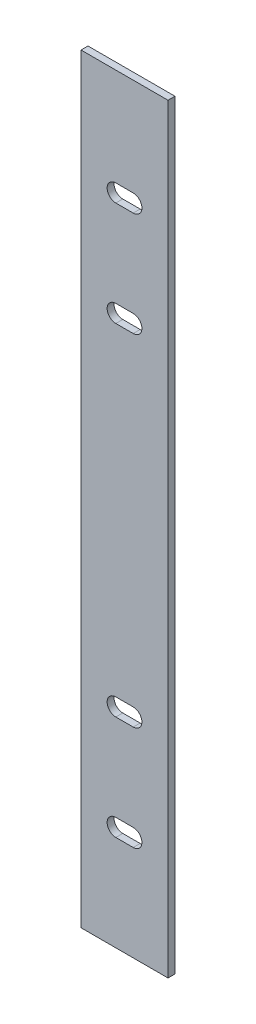
from build123d import *

# Parameters (mm, degrees)
BOSS_EXTRUDE1_DEPTH = 20


with BuildPart() as part:
    # Sketch1 → Boss-Extrude1 (new body)
    with BuildSketch(Plane.XY):
        Polygon((7408.989913804, 2462.985883167), (7408.989913804, 4648.985876948), (7658.989913804, 4648.985876948), (7658.989913804, 2462.985883253), align=None)
        with BuildLine():
            Line((7508.989913506, 4367.985877479), (7558.989913353, 4367.985877479))
            ThreePointArc((7558.989913353, 4367.985877479), (7583.98991328, 4342.985877555), (7558.989913357, 4317.985877628))
            Line((7558.989913357, 4317.985877628), (7508.99011555, 4317.985877628))
            ThreePointArc((7508.99011555, 4317.985877628), (7483.989632688, 4342.98577653), (7508.989913506, 4367.985877479))
        make_face(mode=Mode.SUBTRACT)
        with BuildLine():
            Line((7508.990115362, 3087.985881301), (7558.98932559, 3087.985881301))
            ThreePointArc((7558.98932559, 3087.985881301), (7583.989619399, 3062.986175259), (7558.989913357, 3037.98588145))
            Line((7558.989913357, 3037.98588145), (7508.989913506, 3037.98588145))
            ThreePointArc((7508.989913506, 3037.98588145), (7483.989913645, 3062.985982304), (7508.990115362, 3087.985881301))
        make_face(mode=Mode.SUBTRACT)
        with BuildLine():
            Line((7508.989913506, 4067.985878375), (7558.989913353, 4067.985878375))
            ThreePointArc((7558.989913353, 4067.985878375), (7583.989913278, 4042.985878449), (7558.989913353, 4017.985878524))
            Line((7558.989913353, 4017.985878524), (7508.990115553, 4017.985878524))
            ThreePointArc((7508.990115553, 4017.985878524), (7483.989632674, 4042.985777424), (7508.989913506, 4067.985878375))
        make_face(mode=Mode.SUBTRACT)
        with BuildLine():
            Line((7508.989913506, 2787.985882197), (7558.989325591, 2787.985882197))
            ThreePointArc((7558.989325591, 2787.985882197), (7583.989619399, 2762.986176154), (7558.989913357, 2737.985882346))
            Line((7558.989913357, 2737.985882346), (7508.989913506, 2737.985882346))
            ThreePointArc((7508.989913506, 2737.985882346), (7483.989770854, 2762.985882271), (7508.989913506, 2787.985882197))
        make_face(mode=Mode.SUBTRACT)
    extrude(amount=BOSS_EXTRUDE1_DEPTH)


solid = part.part
